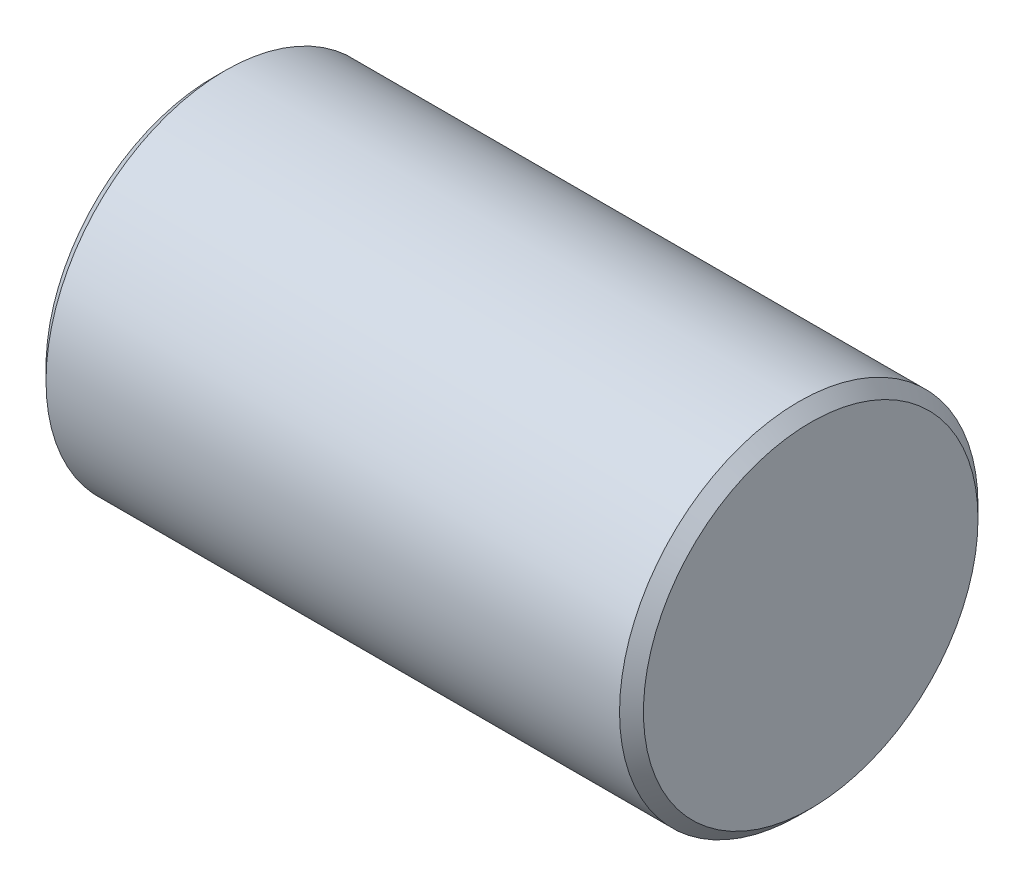
from build123d import *

# Parameters (mm, degrees)
SKETCH_1_R      = 15
EXTRUDE_1_DEPTH = 50
CHAMFER_1_SIZE  = 1


with BuildPart() as part:
    # 草图1 → 凸台-拉伸1 (new body)
    with BuildSketch(Plane(origin=(0, 0, 0), x_dir=(0, 0, -1), z_dir=(1, 0, 0))):
        Circle(SKETCH_1_R)
    extrude(amount=EXTRUDE_1_DEPTH)

    # 倒角1
    chamfer_1_edges = [part.edges().sort_by_distance(p)[0] for p in [
        (0, 0, 15),
        (50, 0, 15),
    ]]
    chamfer(chamfer_1_edges, length=CHAMFER_1_SIZE)


solid = part.part
